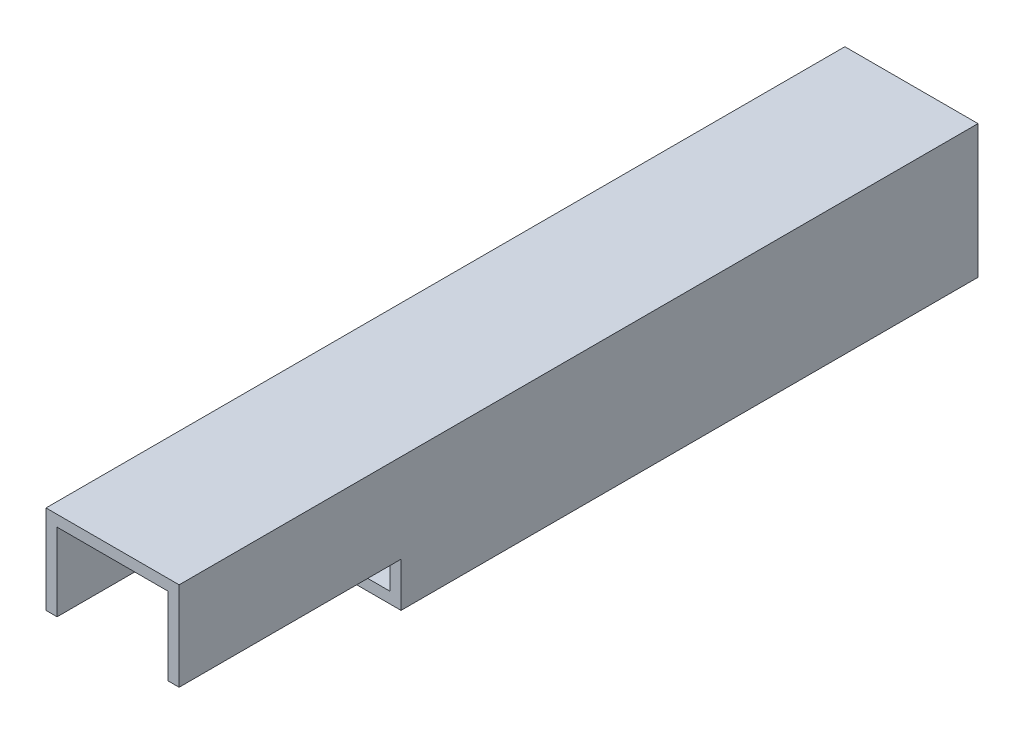
SolidWorks part; units mm, degrees
ref_plane "Front Plane" through (0, 0, 0) normal (0, 0, 1) x (1, 0, 0)
ref_plane "Top Plane" through (0, 0, 0) normal (0, 1, 0) x (1, 0, 0)
ref_plane "Right Plane" through (0, 0, 0) normal (1, 0, 0) x (0, 0, -1)
sketch "Sketch1" plane through (0, 0, 0) normal (0, 0, 1) x (1, 0, 0)
  line L1 (-15, 15) -> (15, 15)
  line L2 (-15, 15) -> (-15, -15)
  line L3 (-15, -15) -> (15, -15)
  line L4 (15, 15) -> (15, -15)
  line L5 (0, -15) -> (0, 15) construction
  line L6 (-15, 0) -> (15, 0) construction
  point P0 (0, 0)
  dimension "D1" = 30
  dimension "D2" = 30
extrude "Boss-Extrude1" add sketch "Sketch1" along normal blind 180
sketch "Sketch2" plane through (0, 0, 180) normal (0, 0, 1) x (1, 0, 0)
  line L1 (-15, 15) -> (15, 15)
  line L2 (-15, 15) -> (-15, -15)
  line L3 (-15, -15) -> (15, -15)
  line L4 (15, 15) -> (15, -15)
  line L5 (0, -15) -> (0, 15) construction
  line L6 (-15, 0) -> (15, 0) construction
  point P0 (0, 0)
  dimension "D1" = 30
  dimension "D2" = 30
sketch "Sketch3" plane through (0, -15, 0) normal (0, -1, 0) x (1, 0, 0)
  line L0 (-15, 130) -> (15, 130)
  line L1 (-15, 180) -> (-15, 0) construction
  line L2 (15, 180) -> (15, 0) construction
  line L3 (15, 180) -> (15, 130)
  dimension "D1" = 50
  dimension "D2" = 30
sketch "Sketch5" plane through (0, 0, 0) normal (0, 0, -1) x (-1, 0, 0)
  line L1 (-12.5, 12.5) -> (12.5, 12.5)
  line L2 (-12.5, 12.5) -> (-12.5, -12.5)
  line L3 (-12.5, -12.5) -> (12.5, -12.5)
  line L4 (12.5, 12.5) -> (12.5, -12.5)
  line L5 (0, -12.5) -> (0, 12.5) construction
  line L6 (-12.5, 0) -> (12.5, 0) construction
  point P0 (0, 0)
  dimension "D1" = 25
  dimension "D2" = 25
extrude "Cut-Extrude4" cut sketch "Sketch5" against normal through all
extrude "Cut-Extrude3" cut sketch "Sketch3" against normal blind 10 and the other way through all flip side to cut
